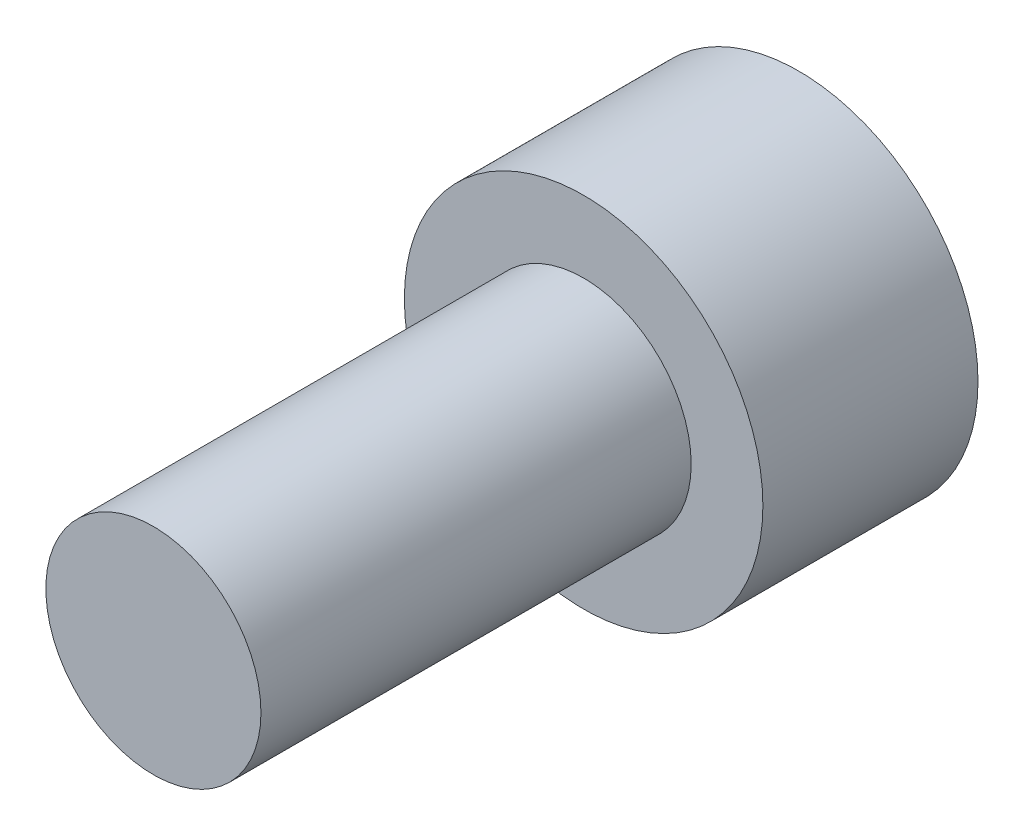
from build123d import *

# Parameters (mm, degrees)
SKETCH1_R           = 2.5
BOSS_EXTRUDE1_DEPTH = 3
SKETCH2_R           = 1.5
BOSS_EXTRUDE2_DEPTH = 6


with BuildPart() as part:
    # Sketch1 → Boss-Extrude1 (new body)
    with BuildSketch(Plane.XY):
        Circle(SKETCH1_R)
    extrude(amount=BOSS_EXTRUDE1_DEPTH)

    # Sketch2 → Boss-Extrude2 (add)
    with BuildSketch(Plane.XY.offset(3)):
        Circle(SKETCH2_R)
    extrude(amount=BOSS_EXTRUDE2_DEPTH)


solid = part.part
